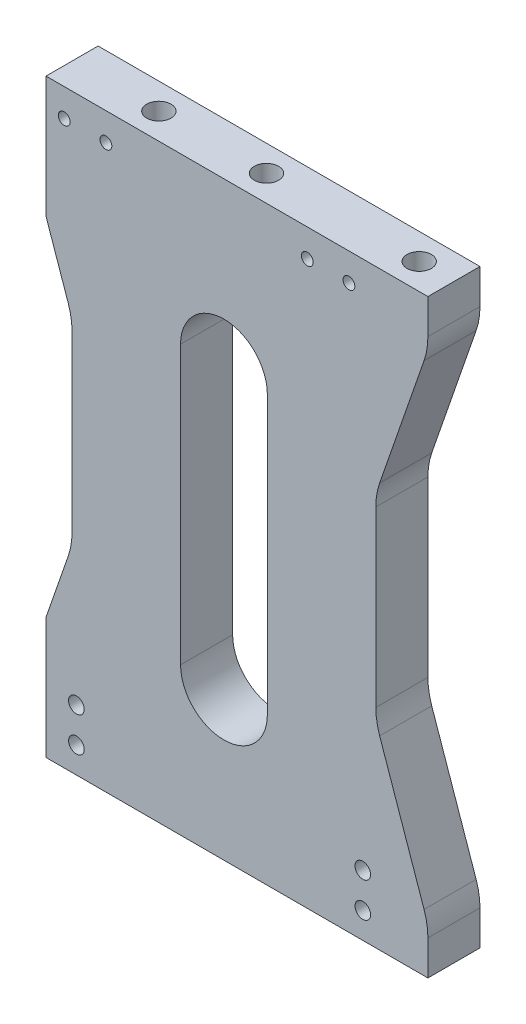
from build123d import *

# Parameters (mm, degrees)
BOSS_EXTRUDE1_DEPTH      = 30
SKETCH4_W                = 15
SKETCH4_H                = 340
CUT_EXTRUDE1_DEPTH       = 415.3971525
M16_TAPPED_HOLE3_D       = 14
M16_TAPPED_HOLE3_DEPTH   = 60
M16_TAPPED_HOLE3_TIP     = 4.206024333
M16_TAPPED_HOLE2_D       = 14
M16_TAPPED_HOLE2_DEPTH   = 50
M16_TAPPED_HOLE2_TIP     = 4.206024333
M8_TAPPED_HOLE1_D        = 6.8
F_9_0_9_DIAMETER_HOLE1_D = 9


with BuildPart() as part:
    # Sketch1 → Boss-Extrude1 (new body)
    with BuildSketch(Plane.XY):
        with BuildLine():
            Line((0, 0), (235, 0))
            Line((235, 0), (235, 20))
            ThreePointArc((235, 20), (234.444340269, 26.644096684), (232.792798963, 33.103600519))
            Line((232.792798963, 33.103600519), (207.207201037, 106.896399481))
            ThreePointArc((207.207201037, 106.896399481), (205.555659731, 113.355903316), (205, 120))
            Line((205, 120), (205, 220))
            ThreePointArc((205, 220), (205.555659731, 226.644096684), (207.207201037, 233.103600519))
            Line((207.207201037, 233.103600519), (232.792798963, 306.896399481))
            ThreePointArc((232.792798963, 306.896399481), (234.444340269, 313.355903316), (235, 320))
            Line((235, 320), (235, 340))
            Line((235, 340), (0, 340))
            Line((0, 340), (0, 320))
            ThreePointArc((0, 320), (0.555659731, 313.355903316), (2.207201037, 306.896399481))
            Line((2.207201037, 306.896399481), (27.792798963, 233.103600519))
            ThreePointArc((27.792798963, 233.103600519), (29.444340269, 226.644096684), (30, 220))
            Line((30, 220), (30, 120))
            ThreePointArc((30, 120), (29.444340269, 113.355903316), (27.792798963, 106.896399481))
            Line((27.792798963, 106.896399481), (2.207201037, 33.103600519))
            ThreePointArc((2.207201037, 33.103600519), (0.555659731, 26.644096684), (0, 20))
            Line((0, 20), (0, 0))
        make_face()
        with BuildLine():
            Line((92.5, 85), (92.5, 245))
            ThreePointArc((92.5, 245), (117.5, 270), (142.5, 245))
            Line((142.5, 245), (142.5, 85))
            ThreePointArc((142.5, 85), (117.5, 60), (92.5, 85))
        make_face(mode=Mode.SUBTRACT)
    extrude(amount=BOSS_EXTRUDE1_DEPTH)

    # Sketch4 → Cut-Extrude1 (cut, through all)
    with BuildSketch(Plane.XY.offset(30)):
        with Locations((7.5, 170)):
            Rectangle(SKETCH4_W, SKETCH4_H)
    extrude(amount=-CUT_EXTRUDE1_DEPTH, mode=Mode.SUBTRACT)

    # M16 Tapped Hole3
    with Locations(Plane(origin=(0, 0, 0), x_dir=(-1, 0, 0), z_dir=(0, -1, 0))):
        with Locations((-215, -15), (-65, -15), (-140, -15)):
            Hole(M16_TAPPED_HOLE3_D / 2, depth=M16_TAPPED_HOLE3_DEPTH)
            with Locations((0, 0, -(M16_TAPPED_HOLE3_DEPTH + M16_TAPPED_HOLE3_TIP / 2))):  # 118° drill point
                Cone(0, M16_TAPPED_HOLE3_D / 2, M16_TAPPED_HOLE3_TIP, mode=Mode.SUBTRACT)

    # M16 Tapped Hole2
    with Locations(Plane(origin=(0, 340, 0), x_dir=(1, 0, 0), z_dir=(0, 1, 0))):
        with Locations((215, -15), (65, -15), (127, -15)):
            Hole(M16_TAPPED_HOLE2_D / 2, depth=M16_TAPPED_HOLE2_DEPTH)
            with Locations((0, 0, -(M16_TAPPED_HOLE2_DEPTH + M16_TAPPED_HOLE2_TIP / 2))):  # 118° drill point
                Cone(0, M16_TAPPED_HOLE2_D / 2, M16_TAPPED_HOLE2_TIP, mode=Mode.SUBTRACT)

    # M8 Tapped Hole1 (through all)
    with Locations(Plane.XY.offset(30)):
        with Locations((25.5, 324), (49.5, 324), (189.5, 324), (165.5, 324)):
            Hole(M8_TAPPED_HOLE1_D / 2)

    # Ø9.0 (9) Diameter Hole1 (through all)
    with Locations(Plane.XY.offset(30)):
        with Locations((197.5, 15), (197.5, 35), (32.5, 15), (32.5, 35)):
            Hole(F_9_0_9_DIAMETER_HOLE1_D / 2)


solid = part.part
